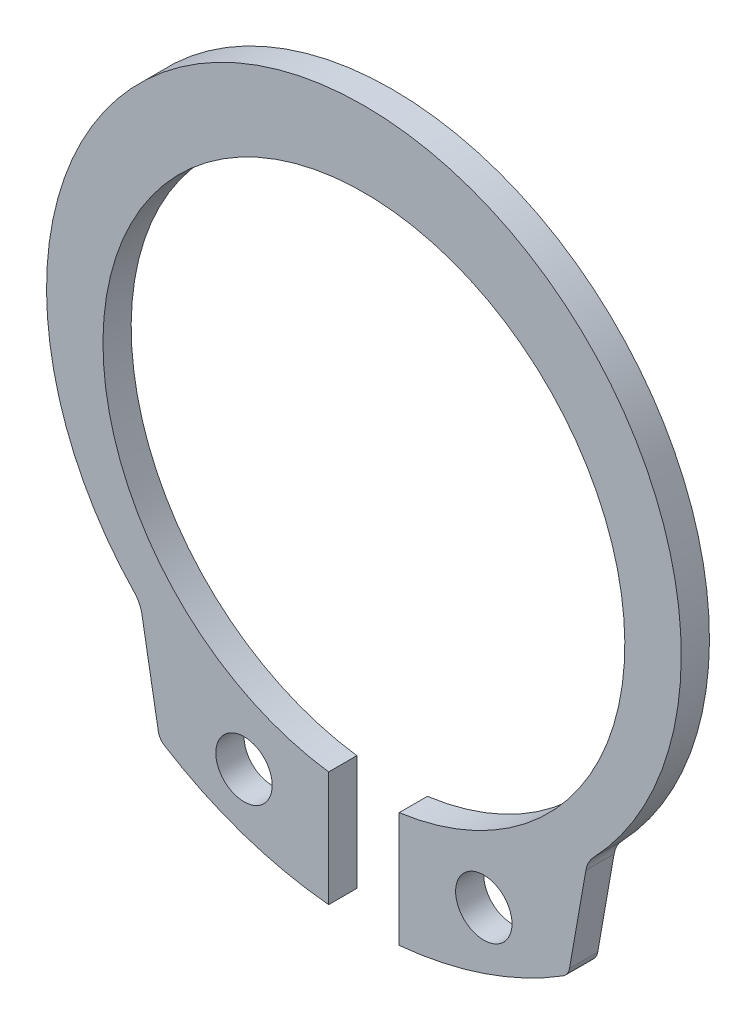
from build123d import *

# Parameters (mm, degrees)
SKETCH_1_R      = 2
EXTRUDE_1_DEPTH = 2


with BuildPart() as part:
    # 草图1 → 凸台-拉伸1 (new body)
    with BuildSketch(Plane.XY):
        with BuildLine():
            Line((-14.576201266, -23.207463353), (-15.742490369, -16.580463555))
            ThreePointArc((-15.742490369, -16.580463555), (-15.927700406, -16.024070615), (-16.26632367, -15.545311649))
            ThreePointArc((-16.26632367, -15.545311649), (0, 22.5), (16.26632367, -15.545311649))
            ThreePointArc((16.26632367, -15.545311649), (15.927700406, -16.024070615), (15.742490369, -16.580463555))
            Line((15.742490369, -16.580463555), (14.576201266, -23.207463353))
            ThreePointArc((14.576201266, -23.207463353), (14.420792767, -23.592708818), (14.122248494, -23.881563776))
            ThreePointArc((14.122248494, -23.881563776), (8.541490175, -26.531326793), (2.5, -27.822258212))
            Line((2.5, -27.822258212), (2.5, -19.67030278))
            ThreePointArc((2.5, -19.67030278), (0, 17.16), (-2.5, -19.67030278))
            Line((-2.5, -19.67030278), (-2.5, -27.822258212))
            ThreePointArc((-2.5, -27.822258212), (-8.541490175, -26.531326793), (-14.122248494, -23.881563776))
            ThreePointArc((-14.122248494, -23.881563776), (-14.420792767, -23.592708818), (-14.576201266, -23.207463353))
        make_face()
        with Locations((-8.5, -22.5)):
            Circle(SKETCH_1_R, mode=Mode.SUBTRACT)
        with Locations((8.5, -22.5)):
            Circle(SKETCH_1_R, mode=Mode.SUBTRACT)
    extrude(amount=EXTRUDE_1_DEPTH)


solid = part.part
